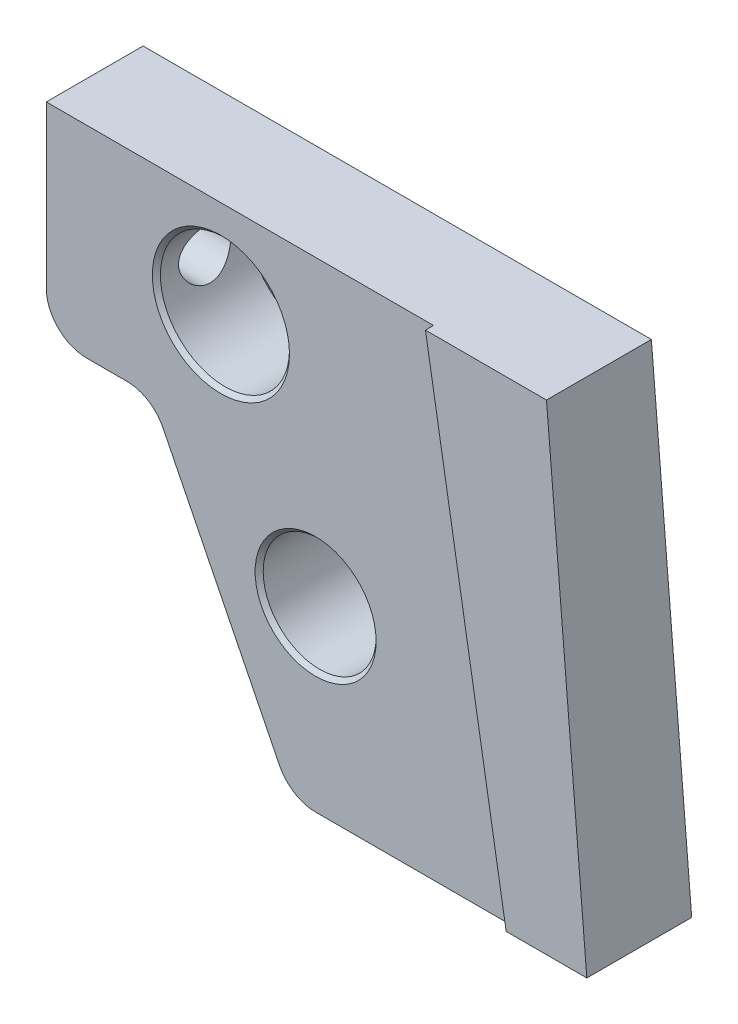
SolidWorks part; units mm, degrees
ref_plane "Front Plane" through (0, 0, 0) normal (0, 0, 1) x (1, 0, 0)
ref_plane "Top Plane" through (0, 0, 0) normal (0, 1, 0) x (1, 0, 0)
ref_plane "Right Plane" through (0, 0, 0) normal (1, 0, 0) x (0, 0, -1)
sketch "Sketch1" plane through (0, 0, 0) normal (0, 0, 1) x (1, 0, 0)
  line L0 (0, 5) -> (0, 25)
  line L1 (0, 25) -> (63, 25)
  line L3 (68, -34.5434) -> (33.3851, -34.5434)
  line L4 (28.9091, -31.7716) -> (14.4732, -2.7718)
  line L5 (9.9971, 0) -> (5, 0)
  line L6 (21.6451, 13) -> (19.4656, 38.9556) construction
  line L7 (63, 25) -> (68, -34.5434)
  line L8 (69.7923, -37.9615) -> (63.0646, 42.1565) construction
  circle A0 centre (21.6451, 13) radius 8
  circle A1 centre (33.3851, -12.47) radius 7
  arc A2 (28.9091, -31.7716) -> (33.3851, -34.5434) centre (33.3851, -29.5434) ccw
  arc A3 (9.9971, 0) -> (14.4732, -2.7718) centre (9.9971, -5) cw
  arc A4 (5, 0) -> (0, 5) centre (5, 5) cw
  circle A6 centre (58.6451, -6.4349) radius 2.5 construction
  point P24 (0, 0)
  dimension "D2" = 4.8
  dimension "D5" = 16
  dimension "D7" = 14
  dimension "D10" = 5
  dimension "D1" = 63
  dimension "D3" = 68
  dimension "D4" = 25.26
  dimension "D6" = 12
  dimension "D8" = 11.74
  dimension "D9" = 25.47
  dimension "D11" = 9.9971
  dimension "D13" = 25
extrude "Boss-Extrude1" add sketch "Sketch1" along normal blind 13
sketch "Sketch2" plane through (0, 0, 13) normal (0, 0, 1) x (1, 0, 0)
  line L0 (48, 25) -> (58, -34.5434)
  line L6 (63, 25) -> (0, 25)
  line L7 (0, 25) -> (0, 5)
  line L8 (5, 0) -> (9.9971, 0)
  line L9 (14.4732, -2.7718) -> (28.9091, -31.7716)
  line L10 (33.3851, -34.5434) -> (68, -34.5434)
  line L11 (68, -34.5434) -> (63, 25)
  line L12 (48, 25) -> (0, 25)
  line L13 (0, 25) -> (0, 5)
  line L14 (5, 0) -> (9.9971, 0)
  line L15 (14.4732, -2.7718) -> (28.9091, -31.7716)
  line L16 (33.3851, -34.5434) -> (58, -34.5434)
  arc A3 (0, 5) -> (5, 0) centre (5, 5) ccw
  arc A4 (14.4732, -2.7718) -> (9.9971, 0) centre (9.9971, -5) ccw
  arc A5 (28.9091, -31.7716) -> (33.3851, -34.5434) centre (33.3851, -29.5434) ccw
  arc A6 (0, 5) -> (5, 0) centre (5, 5) ccw
  arc A7 (14.4732, -2.7718) -> (9.9971, 0) centre (9.9971, -5) ccw
  arc A8 (28.9091, -31.7716) -> (33.3851, -34.5434) centre (33.3851, -29.5434) ccw
  dimension "D2" = 48
  dimension "D3" = 58
  dimension "D1" = 0
extrude "Cut-Extrude1" cut sketch "Sketch2" against normal blind 1
chamfer "Chamfer2" distance 0.5 angle 45 4 edges at (40.3851, -12.47, 12) (29.6451, 13, 12) (29.6451, 13, 0) (40.3851, -12.47, 0)
sketch "Sketch3" plane through (0, 0, 0) normal (-1, 0, 0) x (0, 0, 1)
  line L0 (6, 25) -> (6, 14.4486) construction
  line L1 (12, 25) -> (0, 25) construction
  circle A0 centre (6, 13) radius 3.25
  dimension "D1" = 12
  dimension "D2" = 6.5
extrude "Cut-Extrude2" cut sketch "Sketch3" against normal blind 17
